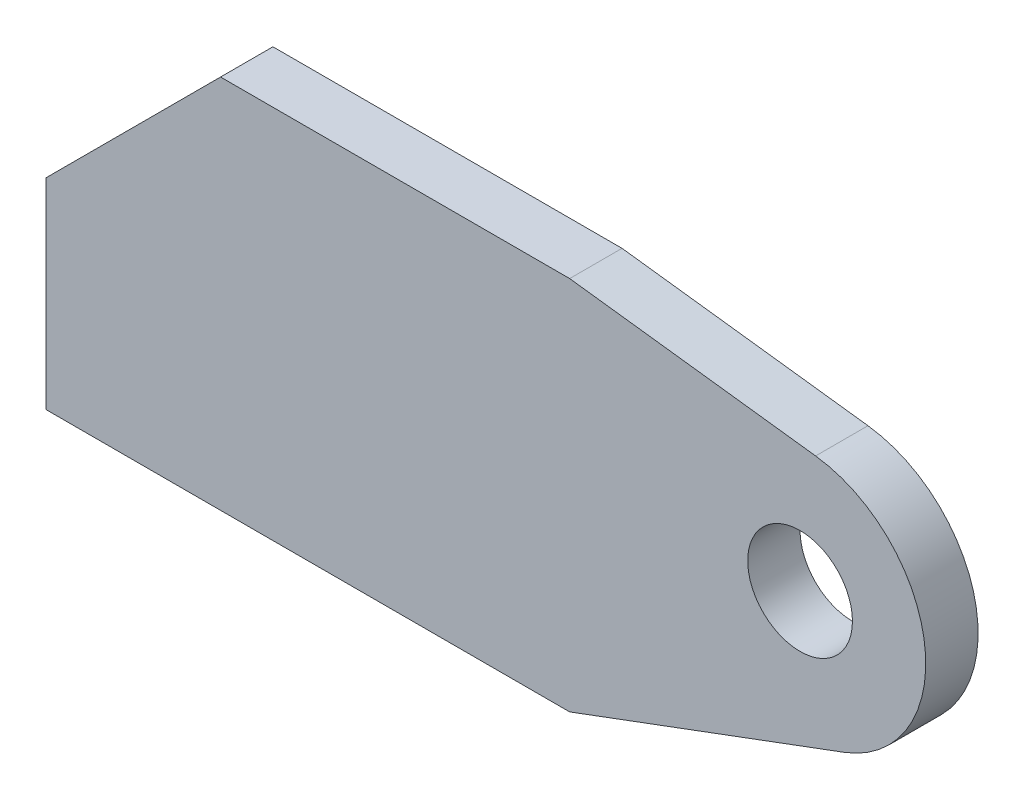
from build123d import *

# Parameters (mm, degrees)
SKETCH1_R           = 30
BOSS_EXTRUDE1_DEPTH = 30


with BuildPart() as part:
    # Sketch1 → Boss-Extrude1 (new body)
    with BuildSketch(Plane.XY):
        with BuildLine():
            Line((0, 0), (300, 0))
            Line((300, 0), (457.131807961, 58.528582136))
            ThreePointArc((457.131807961, 58.528582136), (503.513512073, 134.355692129), (440.900386954, 197.44776492))
            Line((440.900386954, 197.44776492), (300, 215))
            Line((300, 215), (100, 215))
            Line((100, 215), (0, 115))
            Line((0, 115), (0, 0))
        make_face()
        with Locations((432, 126)):
            Circle(SKETCH1_R, mode=Mode.SUBTRACT)
    extrude(amount=BOSS_EXTRUDE1_DEPTH)


solid = part.part
